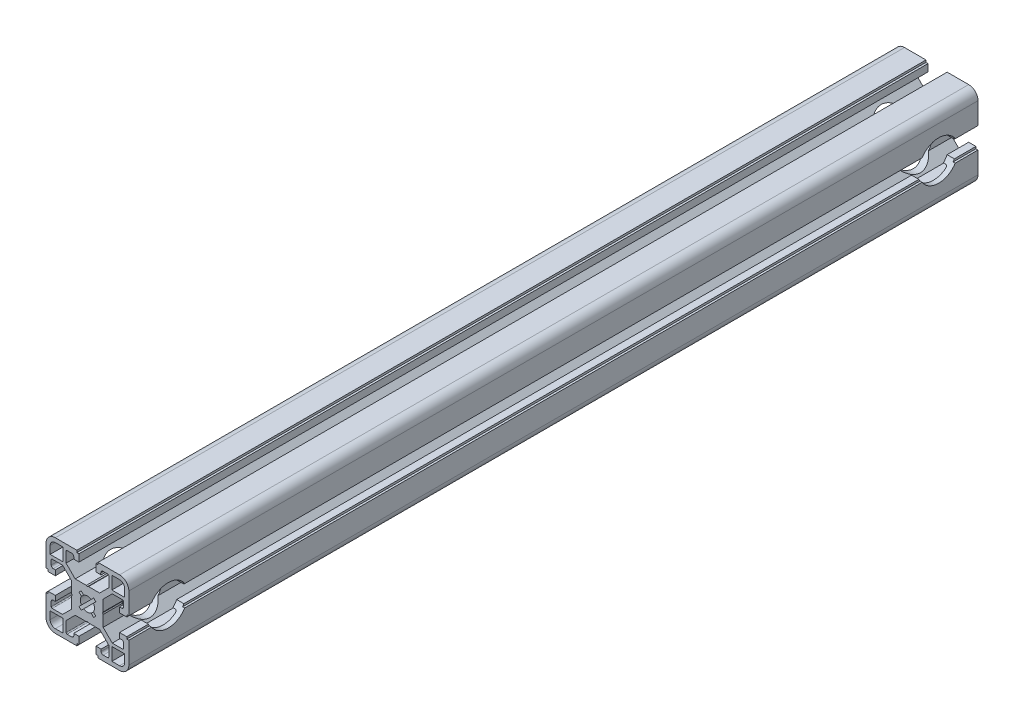
from build123d import *

# Parameters (mm, degrees)
EXTRUDE_1_DEPTH         = 410
HOLE_WIZARD_19_0_19_1_D = 19


with BuildPart() as part:
    # 草图1 → 凸台-拉伸1 (new body)
    with BuildSketch(Plane.XY):
        with BuildLine():
            Line((-18.9995, -4.100341675), (-18.9995, -5.100341675))
            Line((-18.9995, -5.100341675), (-19.9995, -5.100341675))
            Line((-19.9995, -5.100341675), (-19.9995, -15.500341675))
            ThreePointArc((-19.9995, -15.500341675), (-18.681480515, -18.682322191), (-15.4995, -20.000341675))
            Line((-15.4995, -20.000341675), (-5.0995, -20.000341675))
            Line((-5.0995, -20.000341675), (-5.0995, -19.000341675))
            Line((-5.0995, -19.000341675), (-4.0995, -19.000341675))
            Line((-4.0995, -19.000341675), (-4.0995, -15.500341675))
            Line((-4.0995, -15.500341675), (-6.5995, -15.500341675))
            Line((-6.5995, -15.500341675), (-6.5995, -16.500341675))
            ThreePointArc((-6.5995, -16.500341675), (-6.892393219, -17.207448457), (-7.5995, -17.500341675))
            Line((-7.5995, -17.500341675), (-9.7995, -17.500341675))
            ThreePointArc((-9.7995, -17.500341675), (-10.153053391, -17.353895066), (-10.2995, -17.000341675))
            Line((-10.2995, -17.000341675), (-10.2995, -11.997341675))
            Line((-10.2995, -11.997341675), (-5.9025, -7.600341675))
            Line((-5.9025, -7.600341675), (-0.5195, -7.600341675))
            Line((-0.5195, -7.600341675), (0.0005, -7.300341675))
            Line((0.0005, -7.300341675), (0.5195, -7.600341675))
            Line((0.5195, -7.600341675), (5.9035, -7.600341675))
            Line((5.9035, -7.600341675), (10.3005, -11.997341675))
            Line((10.3005, -11.997341675), (10.3005, -17.000341675))
            ThreePointArc((10.3005, -17.000341675), (10.154053391, -17.353895066), (9.8005, -17.500341675))
            Line((9.8005, -17.500341675), (7.6005, -17.500341675))
            ThreePointArc((7.6005, -17.500341675), (6.893393219, -17.207448457), (6.6005, -16.500341675))
            Line((6.6005, -16.500341675), (6.6005, -15.500341675))
            Line((6.6005, -15.500341675), (4.1005, -15.500341675))
            Line((4.1005, -15.500341675), (4.1005, -19.000341675))
            Line((4.1005, -19.000341675), (5.1005, -19.000341675))
            Line((5.1005, -19.000341675), (5.1005, -20.000341675))
            Line((5.1005, -20.000341675), (15.5005, -20.000341675))
            ThreePointArc((15.5005, -20.000341675), (18.682480515, -18.682322191), (20.0005, -15.500341675))
            Line((20.0005, -15.500341675), (20.0005, -5.100341675))
            Line((20.0005, -5.100341675), (19.0005, -5.100341675))
            Line((19.0005, -5.100341675), (19.0005, -4.100341675))
            Line((19.0005, -4.100341675), (15.5005, -4.100341675))
            Line((15.5005, -4.100341675), (15.5005, -6.600341675))
            Line((15.5005, -6.600341675), (16.5005, -6.600341675))
            ThreePointArc((16.5005, -6.600341675), (17.207606781, -6.893234894), (17.5005, -7.600341675))
            Line((17.5005, -7.600341675), (17.5005, -9.800341675))
            ThreePointArc((17.5005, -9.800341675), (17.354053391, -10.153895066), (17.0005, -10.300341675))
            Line((17.0005, -10.300341675), (11.9975, -10.300341675))
            Line((11.9975, -10.300341675), (7.6005, -5.903341675))
            Line((7.6005, -5.903341675), (7.6005, -0.520341675))
            Line((7.6005, -0.520341675), (7.3005, -0.000341675))
            Line((7.3005, -0.000341675), (7.6005, 0.519658325))
            Line((7.6005, 0.519658325), (7.6005, 5.902658325))
            Line((7.6005, 5.902658325), (11.9975, 10.299658325))
            Line((11.9975, 10.299658325), (17.0005, 10.299658325))
            ThreePointArc((17.0005, 10.299658325), (17.354053391, 10.153211715), (17.5005, 9.799658325))
            Line((17.5005, 9.799658325), (17.5005, 7.599658325))
            ThreePointArc((17.5005, 7.599658325), (17.207606781, 6.892551543), (16.5005, 6.599658325))
            Line((16.5005, 6.599658325), (15.5005, 6.599658325))
            Line((15.5005, 6.599658325), (15.5005, 4.099658325))
            Line((15.5005, 4.099658325), (19.0005, 4.099658325))
            Line((19.0005, 4.099658325), (19.0005, 5.099658325))
            Line((19.0005, 5.099658325), (20.0005, 5.099658325))
            Line((20.0005, 5.099658325), (20.0005, 15.499658325))
            ThreePointArc((20.0005, 15.499658325), (18.682480515, 18.68163884), (15.5005, 19.999658325))
            Line((15.5005, 19.999658325), (5.1005, 19.999658325))
            Line((5.1005, 19.999658325), (5.1005, 18.999658325))
            Line((5.1005, 18.999658325), (4.1005, 18.999658325))
            Line((4.1005, 18.999658325), (4.1005, 15.499658325))
            Line((4.1005, 15.499658325), (6.6005, 15.499658325))
            ThreePointArc((6.6005, 15.499658325), (6.393348977, 15.999658325), (6.6005, 16.499658325))
            ThreePointArc((6.6005, 16.499658325), (6.893393219, 17.206765106), (7.6005, 17.499658325))
            Line((7.6005, 17.499658325), (9.8005, 17.499658325))
            ThreePointArc((9.8005, 17.499658325), (10.154053391, 17.353211715), (10.3005, 16.999658325))
            Line((10.3005, 16.999658325), (10.3005, 11.996658325))
            Line((10.3005, 11.996658325), (5.9035, 7.599658325))
            Line((5.9035, 7.599658325), (0.5195, 7.599658325))
            Line((0.5195, 7.599658325), (0.0005, 7.299658325))
            Line((0.0005, 7.299658325), (-0.5195, 7.599658325))
            Line((-0.5195, 7.599658325), (-5.9025, 7.599658325))
            Line((-5.9025, 7.599658325), (-10.2995, 11.996658325))
            Line((-10.2995, 11.996658325), (-10.2995, 16.999658325))
            ThreePointArc((-10.2995, 16.999658325), (-10.153053391, 17.353211715), (-9.7995, 17.499658325))
            Line((-9.7995, 17.499658325), (-7.5995, 17.499658325))
            ThreePointArc((-7.5995, 17.499658325), (-6.892393219, 17.206765106), (-6.5995, 16.499658325))
            Line((-6.5995, 16.499658325), (-6.5995, 15.499658325))
            Line((-6.5995, 15.499658325), (-4.0995, 15.499658325))
            Line((-4.0995, 15.499658325), (-4.0995, 18.999658325))
            Line((-4.0995, 18.999658325), (-5.0995, 18.999658325))
            Line((-5.0995, 18.999658325), (-5.0995, 19.999658325))
            Line((-5.0995, 19.999658325), (-15.4995, 19.999658325))
            ThreePointArc((-15.4995, 19.999658325), (-18.681480515, 18.68163884), (-19.9995, 15.499658325))
            Line((-19.9995, 15.499658325), (-19.9995, 5.099658325))
            Line((-19.9995, 5.099658325), (-18.9995, 5.099658325))
            Line((-18.9995, 5.099658325), (-18.9995, 4.099658325))
            Line((-18.9995, 4.099658325), (-15.4995, 4.099658325))
            Line((-15.4995, 4.099658325), (-15.4995, 6.599658325))
            Line((-15.4995, 6.599658325), (-16.4995, 6.599658325))
            ThreePointArc((-16.4995, 6.599658325), (-17.206606781, 6.892551543), (-17.4995, 7.599658325))
            Line((-17.4995, 7.599658325), (-17.4995, 9.799658325))
            ThreePointArc((-17.4995, 9.799658325), (-17.353053391, 10.153211715), (-16.9995, 10.299658325))
            Line((-16.9995, 10.299658325), (-11.9965, 10.299658325))
            Line((-11.9965, 10.299658325), (-7.5995, 5.902658325))
            Line((-7.5995, 5.902658325), (-7.5995, 0.519658325))
            Line((-7.5995, 0.519658325), (-7.2995, -0.000341675))
            Line((-7.2995, -0.000341675), (-7.5995, -0.520341675))
            Line((-7.5995, -0.520341675), (-7.5995, -5.903341675))
            Line((-7.5995, -5.903341675), (-11.9965, -10.300341675))
            Line((-11.9965, -10.300341675), (-16.9995, -10.300341675))
            ThreePointArc((-16.9995, -10.300341675), (-17.353053391, -10.153895066), (-17.4995, -9.800341675))
            Line((-17.4995, -9.800341675), (-17.4995, -7.600341675))
            ThreePointArc((-17.4995, -7.600341675), (-17.206606781, -6.893234894), (-16.4995, -6.600341675))
            Line((-16.4995, -6.600341675), (-15.4995, -6.600341675))
            Line((-15.4995, -6.600341675), (-15.4995, -4.100341675))
            Line((-15.4995, -4.100341675), (-18.9995, -4.100341675))
        make_face()
        with BuildLine():
            Line((15.5005, -18.000341675), (11.8005, -18.000341675))
            Line((11.8005, -18.000341675), (11.8005, -11.800341675))
            Line((11.8005, -11.800341675), (18.0005, -11.800341675))
            Line((18.0005, -11.800341675), (18.0005, -15.500341675))
            ThreePointArc((18.0005, -15.500341675), (17.268266953, -17.268108628), (15.5005, -18.000341675))
        make_face(mode=Mode.SUBTRACT)
        with BuildLine():
            Line((18.0005, 11.799658325), (11.8005, 11.799658325))
            Line((11.8005, 11.799658325), (11.8005, 17.999658325))
            Line((11.8005, 17.999658325), (15.5005, 17.999658325))
            ThreePointArc((15.5005, 17.999658325), (17.268266953, 17.267425278), (18.0005, 15.499658325))
            Line((18.0005, 15.499658325), (18.0005, 11.799658325))
        make_face(mode=Mode.SUBTRACT)
        with BuildLine():
            Line((-1.8145, -2.875341675), (-3.004391671, -4.066450004))
            Line((-3.004391671, -4.066450004), (-4.065608329, -3.005233346))
            Line((-4.065608329, -3.005233346), (-2.8745, -1.815341675))
            ThreePointArc((-2.8745, -1.815341675), (-3.399473913, -0.000341675), (-2.8745, 1.814658325))
            Line((-2.8745, 1.814658325), (-4.064391671, 3.005766654))
            Line((-4.064391671, 3.005766654), (-3.004391671, 4.065766654))
            Line((-3.004391671, 4.065766654), (-1.8145, 2.874658325))
            ThreePointArc((-1.8145, 2.874658325), (0, 3.399316649), (1.8145, 2.874658325))
            Line((1.8145, 2.874658325), (3.0055, 4.065658325))
            Line((3.0055, 4.065658325), (4.066608329, 3.004549996))
            Line((4.066608329, 3.004549996), (2.8755, 1.814658325))
            ThreePointArc((2.8755, 1.814658325), (3.400473913, -0.000341675), (2.8755, -1.815341675))
            Line((2.8755, -1.815341675), (4.066608329, -3.005233346))
            Line((4.066608329, -3.005233346), (3.0055, -4.066341675))
            Line((3.0055, -4.066341675), (1.8145, -2.875341675))
            ThreePointArc((1.8145, -2.875341675), (0, -3.4), (-1.8145, -2.875341675))
        make_face(mode=Mode.SUBTRACT)
        with BuildLine():
            Line((-17.9995, -15.500341675), (-17.9995, -11.800341675))
            Line((-17.9995, -11.800341675), (-11.7995, -11.800341675))
            Line((-11.7995, -11.800341675), (-11.7995, -18.000341675))
            Line((-11.7995, -18.000341675), (-15.4995, -18.000341675))
            ThreePointArc((-15.4995, -18.000341675), (-17.267266953, -17.268108628), (-17.9995, -15.500341675))
        make_face(mode=Mode.SUBTRACT)
        with BuildLine():
            Line((-11.7995, 17.999658325), (-11.7995, 11.799658325))
            Line((-11.7995, 11.799658325), (-17.9995, 11.799658325))
            Line((-17.9995, 11.799658325), (-17.9995, 15.499658325))
            ThreePointArc((-17.9995, 15.499658325), (-17.267266953, 17.267425278), (-15.4995, 17.999658325))
            Line((-15.4995, 17.999658325), (-11.7995, 17.999658325))
        make_face(mode=Mode.SUBTRACT)
    extrude(amount=-EXTRUDE_1_DEPTH)

    # Ø19.0 (19) 直径孔1 (through all)
    with Locations(Plane(origin=(20.0005, 0, 0), x_dir=(0, 0, -1), z_dir=(1, 0, 0))):
        with Locations((18.999999997, -0.000341675), (391, -0.000341675)):
            Hole(HOLE_WIZARD_19_0_19_1_D / 2)


solid = part.part
